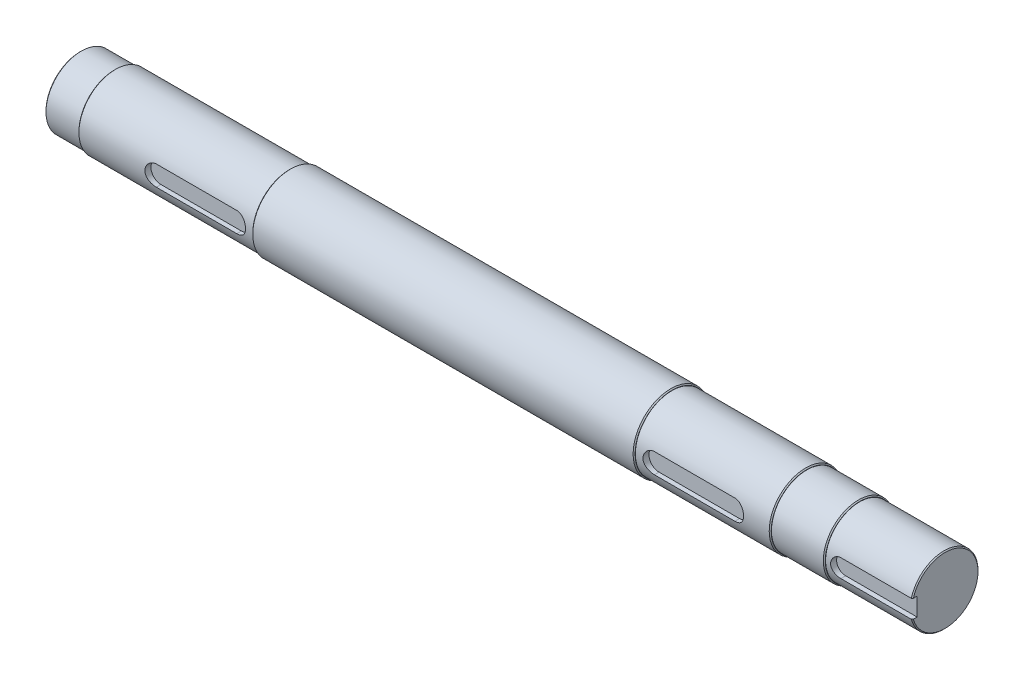
from build123d import *

# Parameters (mm, degrees)
CUT_EXTRUDE1_DEPTH = 12
CUT_EXTRUDE2_DEPTH = 12
CHAMFER1_SIZE      = 2


with BuildPart() as part:
    # Sketch1 → Revolve1 (revolve)
    with BuildSketch(Plane.XY, mode=Mode.PRIVATE) as revolve1_sk:
        Polygon((-796, 70), (-728, 70), (-728, 72.5), (-380, 72.5), (-380, 75), (380, 75), (380, 72.5), (648, 72.5), (648, 70), (753, 70), (753, 67.5), (923, 67.5), (923, 0), (-796, 0), align=None)
    revolve(revolve1_sk.sketch.rotate(Axis((-820.662631097, 0, 0), (1, 0, 0)), 90), axis=Axis((-820.662631097, 0, 0), (1, 0, 0)))

    # Sketch2 → Cut-Extrude1 (cut)
    with BuildSketch(Plane.XY.offset(67.5)):
        with BuildLine():
            Line((923, -18), (781, -18))
            ThreePointArc((781, -18), (763, 0), (781, 18))
            Line((781, 18), (923, 18))
            Line((923, 18), (923, 0))
            Line((923, 0), (923, -18))
        make_face()
    extrude(amount=-CUT_EXTRUDE1_DEPTH, mode=Mode.SUBTRACT)

    # Sketch3 → Cut-Extrude2 (cut)
    with BuildSketch(Plane.XY.offset(72.5)):
        with BuildLine():
            Line((-575, -20), (-415, -20))
            ThreePointArc((-415, -20), (-395, 0), (-415, 20))
            Line((-415, 20), (-575, 20))
            ThreePointArc((-575, 20), (-595, 0), (-575, -20))
        make_face()
        with BuildLine():
            Line((575, 20), (415, 20))
            ThreePointArc((415, 20), (395, 0), (415, -20))
            Line((415, -20), (575, -20))
            ThreePointArc((575, -20), (595, 0), (575, 20))
        make_face()
    extrude(amount=-CUT_EXTRUDE2_DEPTH, mode=Mode.SUBTRACT)

    # Chamfer1
    chamfer1_edges = [part.edges().sort_by_distance(p)[0] for p in [
        (-796, 0, -70),
        (-728, 0, -72.5),
        (-380, 0, -75),
        (380, 0, -75),
        (648, 0, -72.5),
        (753, 0, -70),
        (923, 0, -67.5),
    ]]
    chamfer(chamfer1_edges, length=CHAMFER1_SIZE)


solid = part.part
